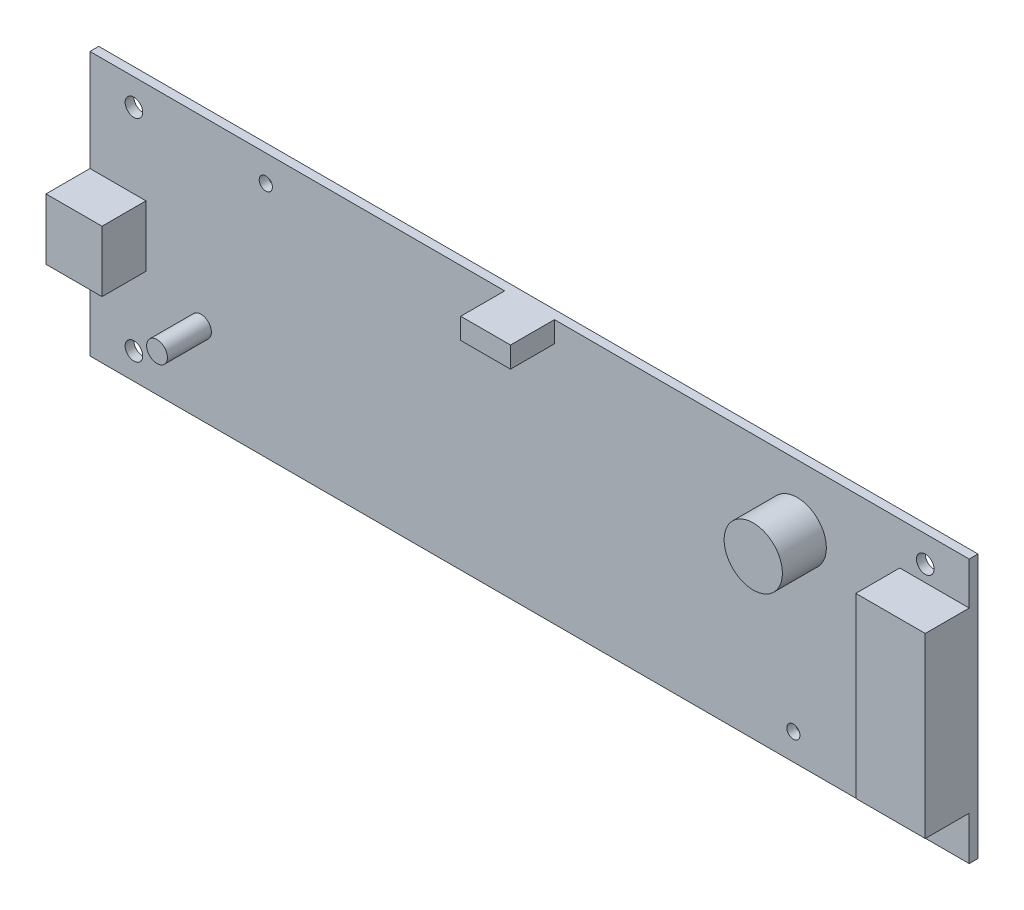
from build123d import *

# Parameters (mm, degrees)
SKETCH1_W           = 100
SKETCH1_H           = 30
SKETCH1_R           = 1
BOSS_EXTRUDE1_DEPTH = 1
SKETCH2_R           = 3.312148645
SKETCH2_R_2         = 1.182707094
SKETCH2_W           = 7.897065894
SKETCH2_H           = 20.201539664
SKETCH2_W_2         = 5.658967966
SKETCH2_H_2         = 2.382698796
SKETCH2_W_3         = 6.371052581
SKETCH2_H_3         = 6.939357654
BOSS_EXTRUDE2_DEPTH = 5
SKETCH3_W           = 5
SKETCH3_H           = 5
BOSS_EXTRUDE3_DEPTH = 1
SKETCH4_R           = 1
BOSS_EXTRUDE4_DEPTH = 1
SKETCH5_R           = 0.75
CUT_EXTRUDE1_DEPTH  = 10


with BuildPart() as part:
    # Sketch1 → Boss-Extrude1 (new body)
    with BuildSketch(Plane.XY):
        Rectangle(SKETCH1_W, SKETCH1_H)
        with Locations((-45, -12)):
            Circle(SKETCH1_R, mode=Mode.SUBTRACT)
        with Locations((-45, 12)):
            Circle(SKETCH1_R, mode=Mode.SUBTRACT)
        with Locations((45, 12)):
            Circle(SKETCH1_R, mode=Mode.SUBTRACT)
        with Locations((45, -12)):
            Circle(SKETCH1_R, mode=Mode.SUBTRACT)
    extrude(amount=BOSS_EXTRUDE1_DEPTH)

    # Sketch2 → Boss-Extrude2 (add)
    with BuildSketch(Plane.XY.offset(1)):
        with Locations((30.440398969, 7.974336126)):
            Circle(SKETCH2_R)
        with Locations((-37.372165455, -5.749563916)):
            Circle(SKETCH2_R_2)
        with Locations((46.051467053, 0.07257894)):
            Rectangle(SKETCH2_W, SKETCH2_H)
        with Locations((0, 13.808650602)):
            Rectangle(SKETCH2_W_2, SKETCH2_H_2)
        with Locations((-46.814473709, 0)):
            Rectangle(SKETCH2_W_3, SKETCH2_H_3)
    extrude(amount=BOSS_EXTRUDE2_DEPTH)

    # Sketch3 → Boss-Extrude3 (add)
    with BuildSketch(Plane(origin=(0, 0, 0), x_dir=(-1, 0, 0), z_dir=(0, 0, -1))):
        with Locations((-12.5, -7)):
            Rectangle(SKETCH3_W, SKETCH3_H)
        with Locations((-37.5, -7)):
            Rectangle(SKETCH3_W, SKETCH3_H)
        with Locations((37.5, -7)):
            Rectangle(SKETCH3_W, SKETCH3_H)
        with Locations((12.5, -7)):
            Rectangle(SKETCH3_W, SKETCH3_H)
    extrude(amount=BOSS_EXTRUDE3_DEPTH)

    # Sketch4 → Boss-Extrude4 (add)
    with BuildSketch(Plane(origin=(0, 0, -1), x_dir=(-1, 0, 0), z_dir=(0, 0, -1))):
        with Locations((-37.5, -7)):
            Circle(SKETCH4_R)
        with Locations((-12.5, -7)):
            Circle(SKETCH4_R)
        with Locations((12.5, -7)):
            Circle(SKETCH4_R)
        with Locations((37.5, -7)):
            Circle(SKETCH4_R)
    extrude(amount=BOSS_EXTRUDE4_DEPTH)

    # Sketch5 → Cut-Extrude1 (cut)
    with BuildSketch(Plane.XY.offset(1)):
        with Locations((30, -12)):
            Circle(SKETCH5_R)
        with Locations((-30, 12)):
            Circle(SKETCH5_R)
    extrude(amount=-CUT_EXTRUDE1_DEPTH, mode=Mode.SUBTRACT)


solid = part.part
